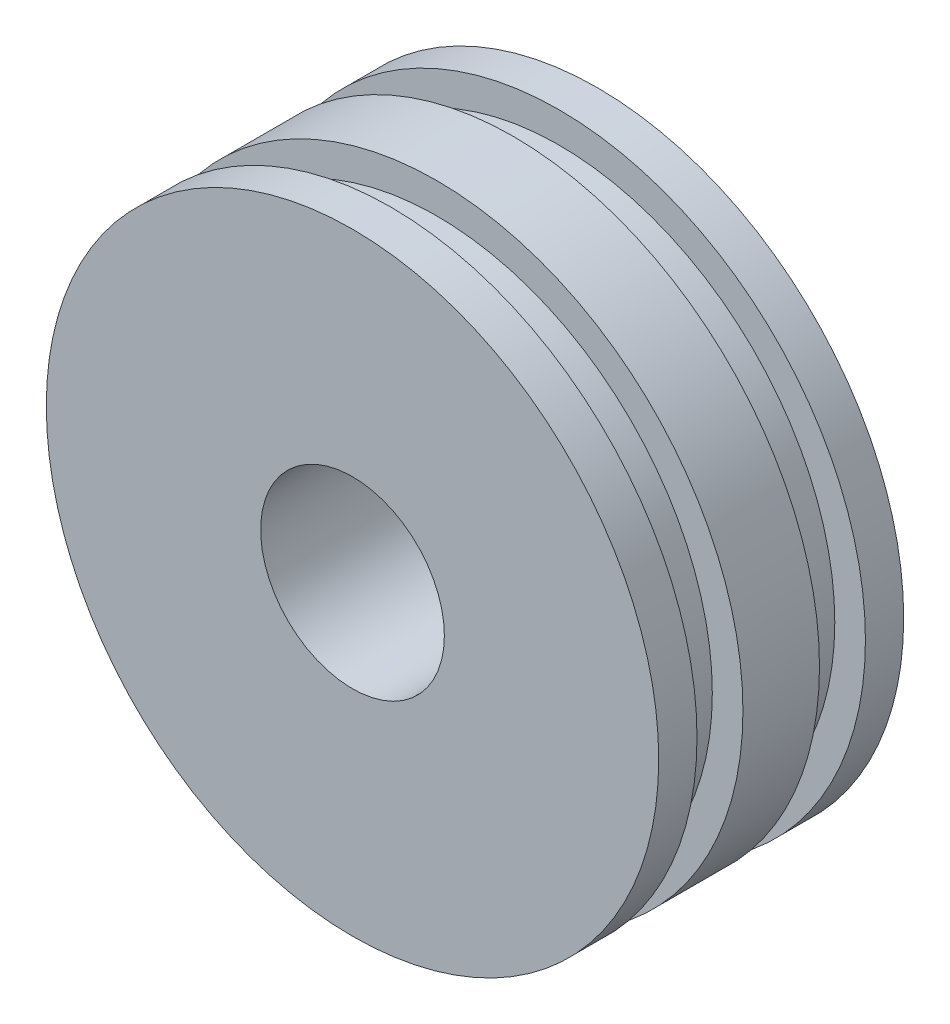
SolidWorks part; units mm, degrees
ref_plane "前视基准面" through (0, 0, 0) normal (0, 0, 1) x (1, 0, 0)
ref_plane "上视基准面" through (0, 0, 0) normal (0, 1, 0) x (1, 0, 0)
ref_plane "右视基准面" through (0, 0, 0) normal (1, 0, 0) x (0, 0, -1)
other "Configuration Table"
sketch "草图1" plane through (0, 0, 0) normal (0, 0, 1) x (1, 0, 0)
  circle A0 centre (0, 0) radius 30
  circle A1 centre (0, 0) radius 100
  dimension "D1" = 60
  dimension "D2" = 200
extrude "凸台-拉伸1" add sketch "草图1" along normal mid plane 80
ref_plane "基准面1" through (0, 0, 20) normal (0, 0, 1) x (1, 0, 0)
sketch "草图2" plane through (0, 0, 20) normal (0, 0, 1) x (1, 0, 0)
  circle A0 centre (0, 0) radius 100 construction
  circle A1 centre (0, 0) radius 100
  circle A2 centre (0, 0) radius 90
  dimension "D1" = 180
extrude "切除-拉伸1" cut sketch "草图2" along normal mid plane 15
mirror "镜向1" about plane through (0, 0, 0) normal (0, 0, 1) of "切除-拉伸1"
